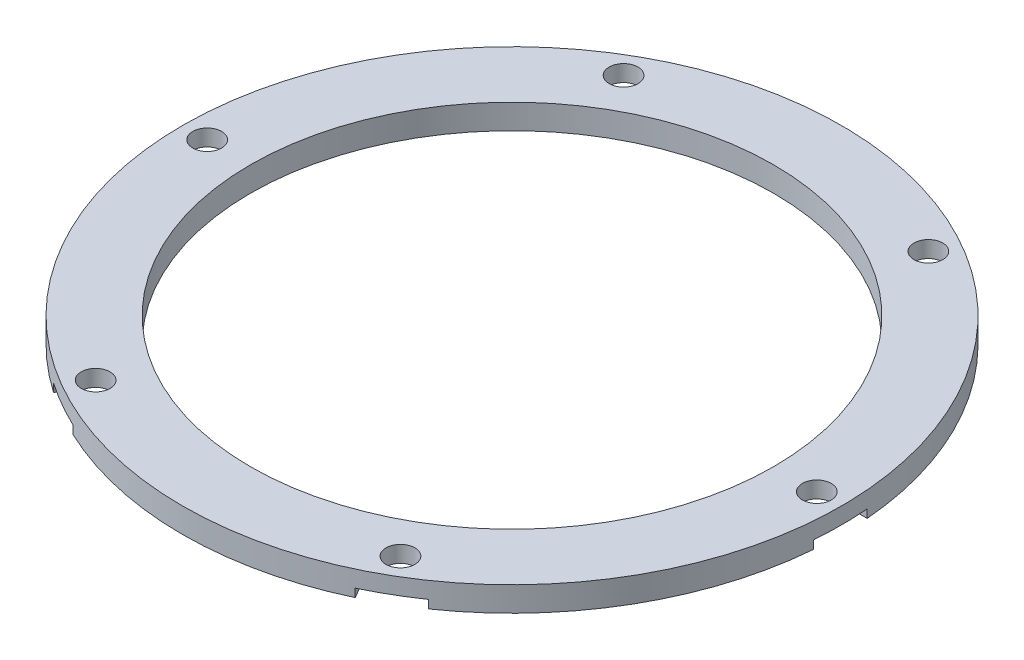
from build123d import *

# Parameters (mm, degrees)
SKETCH1_R           = 40
SKETCH1_R_2         = 31.75
BOSS_EXTRUDE1_DEPTH = 3
SKETCH3_R           = 1.75
CUT_EXTRUDE2_DEPTH  = 57.648036153
CIRPATTERN1_COUNT   = 6
SKETCH5_R           = 3.25
CUT_EXTRUDE4_DEPTH  = 1
CIRPATTERN2_COUNT   = 6
SKETCH6_W           = 3.5
SKETCH6_H           = 6.5
CUT_EXTRUDE5_DEPTH  = 1
CIRPATTERN3_COUNT   = 6


with BuildPart() as part:
    # Sketch1 → Boss-Extrude1 (new body)
    with BuildSketch(Plane(origin=(0, 0, 0), x_dir=(1, 0, 0), z_dir=(0, 1, 0))):
        with Locations(Location((0, 0, 0), (0, 0, 270))):
            Circle(SKETCH1_R)
        with Locations(Location((0, 0, 0), (0, 0, 270))):
            Circle(SKETCH1_R_2, mode=Mode.SUBTRACT)
    extrude(amount=BOSS_EXTRUDE1_DEPTH)

    # Sketch3 → Cut-Extrude2 (cut, through all)
    with BuildSketch(Plane.XZ):
        with Locations(Location((37, 0, 0), (0, 0, 270))):
            Circle(SKETCH3_R)
    cut_extrude2 = extrude(amount=-CUT_EXTRUDE2_DEPTH, mode=Mode.SUBTRACT)

    # CirPattern1: Cut-Extrude2 ×6 about axis
    cirpattern1_axis = Axis((0, 0, 0), (0, 1, 0))
    for i in range(1, CIRPATTERN1_COUNT):
        add(cut_extrude2.rotate(cirpattern1_axis, i * 360 / CIRPATTERN1_COUNT), mode=Mode.SUBTRACT)

    # Sketch5 → Cut-Extrude4 (cut)
    with BuildSketch(Plane.XZ):
        with Locations((18.5, 32.04293994)):
            Circle(SKETCH5_R)
    cut_extrude4 = extrude(amount=-CUT_EXTRUDE4_DEPTH, mode=Mode.SUBTRACT)

    # CirPattern2: Cut-Extrude4 ×6 about axis
    cirpattern2_axis = Axis((0, 0, 0), (0, 1, 0))
    for i in range(1, CIRPATTERN2_COUNT):
        add(cut_extrude4.rotate(cirpattern2_axis, i * 360 / CIRPATTERN2_COUNT), mode=Mode.SUBTRACT)

    # Sketch6 → Cut-Extrude5 (cut)
    with BuildSketch(Plane.XZ):
        with Locations((38.75, 0)):
            Rectangle(SKETCH6_W, SKETCH6_H)
    cut_extrude5 = extrude(amount=-CUT_EXTRUDE5_DEPTH, mode=Mode.SUBTRACT)

    # CirPattern3: Cut-Extrude5 ×6 about axis
    cirpattern3_axis = Axis((0, 0, 0), (0, 1, 0))
    for i in range(1, CIRPATTERN3_COUNT):
        add(cut_extrude5.rotate(cirpattern3_axis, i * 360 / CIRPATTERN3_COUNT), mode=Mode.SUBTRACT)


solid = part.part
